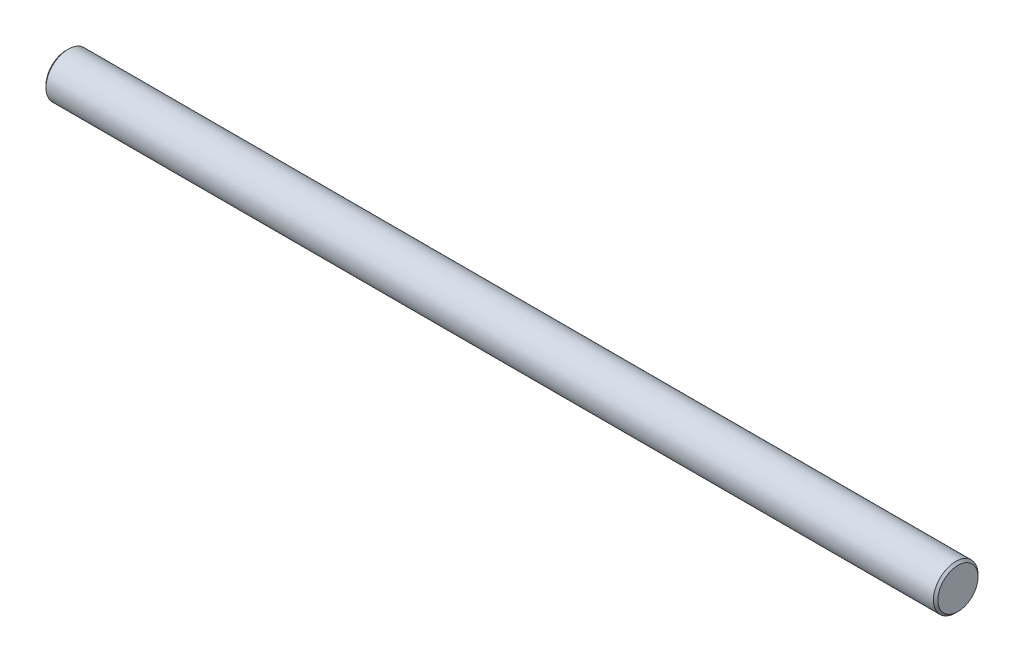
SolidWorks part; units mm, degrees
material "AISI 304"
ref_plane "前视基准面" through (0, 0, 0) normal (0, 0, 1) x (1, 0, 0)
ref_plane "上视基准面" through (0, 0, 0) normal (0, 1, 0) x (1, 0, 0)
ref_plane "右视基准面" through (0, 0, 0) normal (1, 0, 0) x (0, 0, -1)
sketch "草图1" plane through (0, 0, 0) normal (1, 0, 0) x (0, 0, -1)
  circle A0 centre (0, 0) radius 1.5
  dimension "D1" = 3
extrude "凸台-拉伸1" add sketch "草图1" along normal mid plane 60
chamfer "C0.15 倒角1" distance 0.15 angle 45 2 edges at (-30, 0, -1.5) (30, 0, -1.5)
sketch "轴心" plane through (0, 0, 0) normal (1, 0, 0) x (0, 0, -1)
  point P0 (0, 0)
